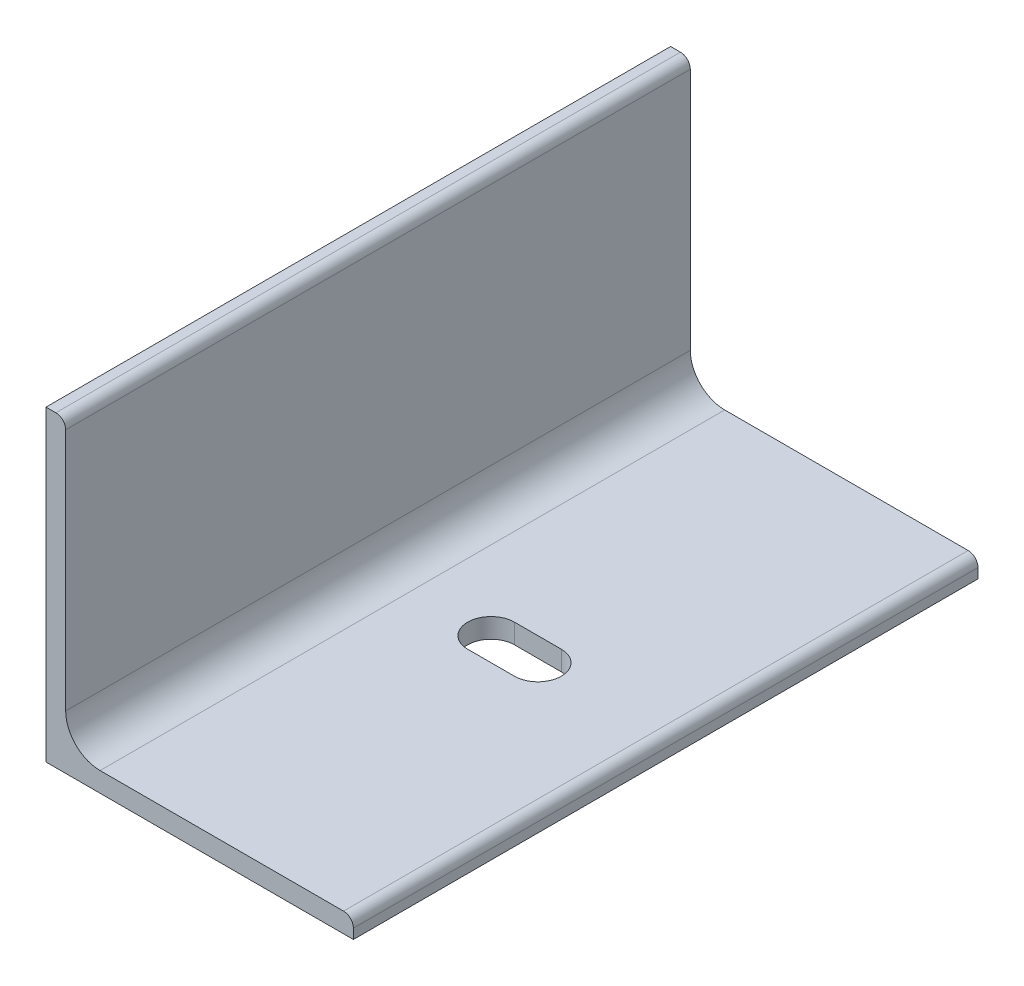
SolidWorks part; units mm, degrees
material "普通碳钢"
ref_plane "Front Plane" through (0, 0, 0) normal (0, 0, 1) x (1, 0, 0)
ref_plane "Top Plane" through (0, 0, 0) normal (0, 1, 0) x (1, 0, 0)
ref_plane "Right Plane" through (0, 0, 0) normal (1, 0, 0) x (0, 0, -1)
sketch "Sketch1" plane through (0, 0, 0) normal (0, 0, 1) x (1, 0, 0)
  line L0 (0, 125) -> (0, 0)
  line L1 (0, 0) -> (125, 0)
  line L2 (8, 121) -> (8, 22)
  line L3 (22, 8) -> (121, 8)
  line L4 (0, 125) -> (4, 125)
  line L5 (125, 0) -> (125, 4)
  arc A0 (4, 125) -> (8, 121) centre (4, 121) cw
  arc A1 (125, 4) -> (121, 8) centre (121, 4) ccw
  arc A2 (8, 22) -> (22, 8) centre (22, 22) ccw
  dimension "D4" = 4
  dimension "D5" = 14
  dimension "D1" = 125
  dimension "D2" = 8
  dimension "D3" = 8
  dimension "D6" = 125
extrude "Boss-Extrude1" add sketch "Sketch1" along normal mid plane 254
sketch "Sketch2" plane through (0, 8, 0) normal (0, 1, 0) x (1, 0, 0)
  line L0 (53.975, 0) -> (73.025, 0) construction
  line L1 (53.975, 9.525) -> (73.025, 9.525)
  line L2 (53.975, -9.525) -> (73.025, -9.525)
  line L4 (-23.7451, 0) -> (140.473, 0) construction
  line L5 (0, -127) -> (0, 127) construction
  arc A0 (53.975, 9.525) -> (53.975, -9.525) centre (53.975, 0) ccw
  arc A1 (73.025, -9.525) -> (73.025, 9.525) centre (73.025, 0) ccw
  point P2 (63.5, 0)
  dimension "D3" = 19.05
  dimension "D1" = 63.5
  dimension "D2" = 19.05
extrude "Cut-Extrude1" cut sketch "Sketch2" against normal blind 304.8
